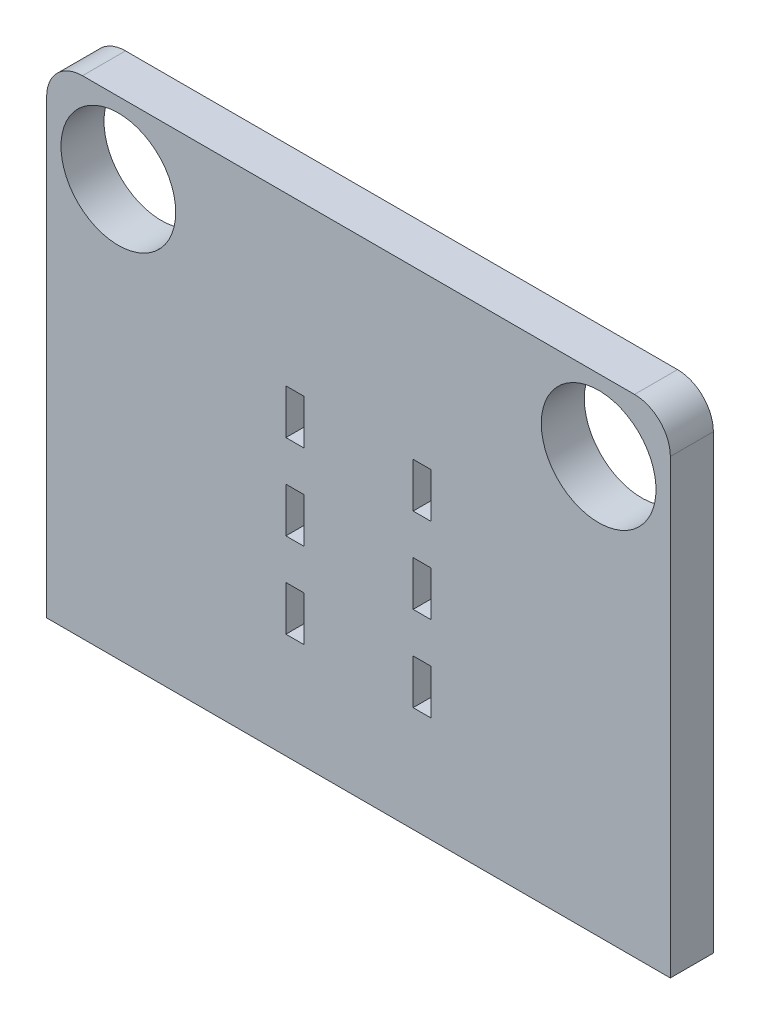
SolidWorks part; units mm, degrees
ref_plane "前视基准面" through (0, 0, 0) normal (0, 0, 1) x (1, 0, 0)
ref_plane "上视基准面" through (0, 0, 0) normal (0, 1, 0) x (1, 0, 0)
ref_plane "右视基准面" through (0, 0, 0) normal (1, 0, 0) x (0, 0, -1)
other "Configuration Table"
sketch "草图1" plane through (0, 0, 0) normal (0, 0, 1) x (1, 0, 0)
  line L0 (-102.769, 1.6599) -> (105.2237, 1.6599) construction
  line L1 (-22.665, 82.5004) -> (-22.665, -82.3366) construction
  line L3 (-109.665, 69.6599) -> (-109.665, -66.3401)
  line L6 (64.335, 69.6599) -> (64.335, -66.3401)
  line L7 (-89.665, 65.6599) -> (-102.769, 65.6599) construction
  line L8 (-37.915, 59.0163) -> (-37.915, -37.8114) construction
  line L9 (-37.915, 23.1025) -> (-42.915, 23.1025)
  line L10 (-42.915, 23.1025) -> (-42.915, 10.6025)
  line L11 (-42.915, 10.6025) -> (-37.915, 10.6025)
  line L12 (-37.915, -0.6475) -> (-42.915, -0.6475)
  line L13 (-42.915, -0.6475) -> (-42.915, -13.1475)
  line L14 (-42.915, -13.1475) -> (-37.915, -13.1475)
  line L15 (-37.915, -24.3975) -> (-42.915, -24.3975)
  line L16 (-42.915, -24.3975) -> (-42.915, -36.8975)
  line L17 (-42.915, -36.8975) -> (-37.915, -36.8975)
  line L18 (-37.915, 23.1025) -> (-37.915, 10.6025)
  line L19 (-37.915, -0.6475) -> (-37.915, -13.1475)
  line L20 (-37.915, -24.3975) -> (-37.915, -36.8975)
  line L21 (-7.415, -24.3975) -> (-2.415, -24.3975)
  line L22 (-2.415, -24.3975) -> (-2.415, -36.8975)
  line L23 (-2.415, -36.8975) -> (-7.415, -36.8975)
  line L24 (-7.415, -24.3975) -> (-7.415, -36.8975)
  line L25 (-7.415, -0.6475) -> (-2.415, -0.6475)
  line L26 (-2.415, -0.6475) -> (-2.415, -13.1475)
  line L27 (-2.415, -13.1475) -> (-7.415, -13.1475)
  line L28 (-7.415, -0.6475) -> (-7.415, -13.1475)
  line L29 (-7.415, 23.1025) -> (-2.415, 23.1025)
  line L30 (-2.415, 23.1025) -> (-2.415, 10.6025)
  line L31 (-2.415, 10.6025) -> (-7.415, 10.6025)
  line L32 (-7.415, 23.1025) -> (-7.415, 10.6025)
  line L33 (-105.665, 49.6599) -> (-105.665, 63.0476) construction
  line L34 (-109.665, 69.6599) -> (64.335, 69.6599)
  line L35 (-109.665, -66.3401) -> (64.335, -66.3401)
  circle A2 centre (-89.665, 49.6599) radius 16
  circle A3 centre (44.335, 49.6599) radius 16
  point P9 (-22.665, 69.6599)
  point P10 (64.335, 1.6599)
  point P11 (-109.665, 1.6599)
  point P31 (-40.415, -0.6475)
  point P34 (-40.415, -24.3975)
  point P47 (-22.665, 69.6599)
  dimension "D3" = 67
  dimension "D4" = 4
  dimension "D1" = 87
  dimension "D2" = 4
  dimension "D6" = 15.25
  dimension "D7" = 5
  dimension "D8" = 12.5
  dimension "D9" = 5
  dimension "D10" = 12.5
  dimension "D11" = 5
  dimension "D12" = 12.5
  dimension "D13" = 11.25
  dimension "D14" = 11.25
extrude "凸台-拉伸1" add sketch "草图1" along normal blind 12
fillet "圆角2" radius 10 2 edges at (64.335, 69.6599, 6) (-109.665, 69.6599, 6)
